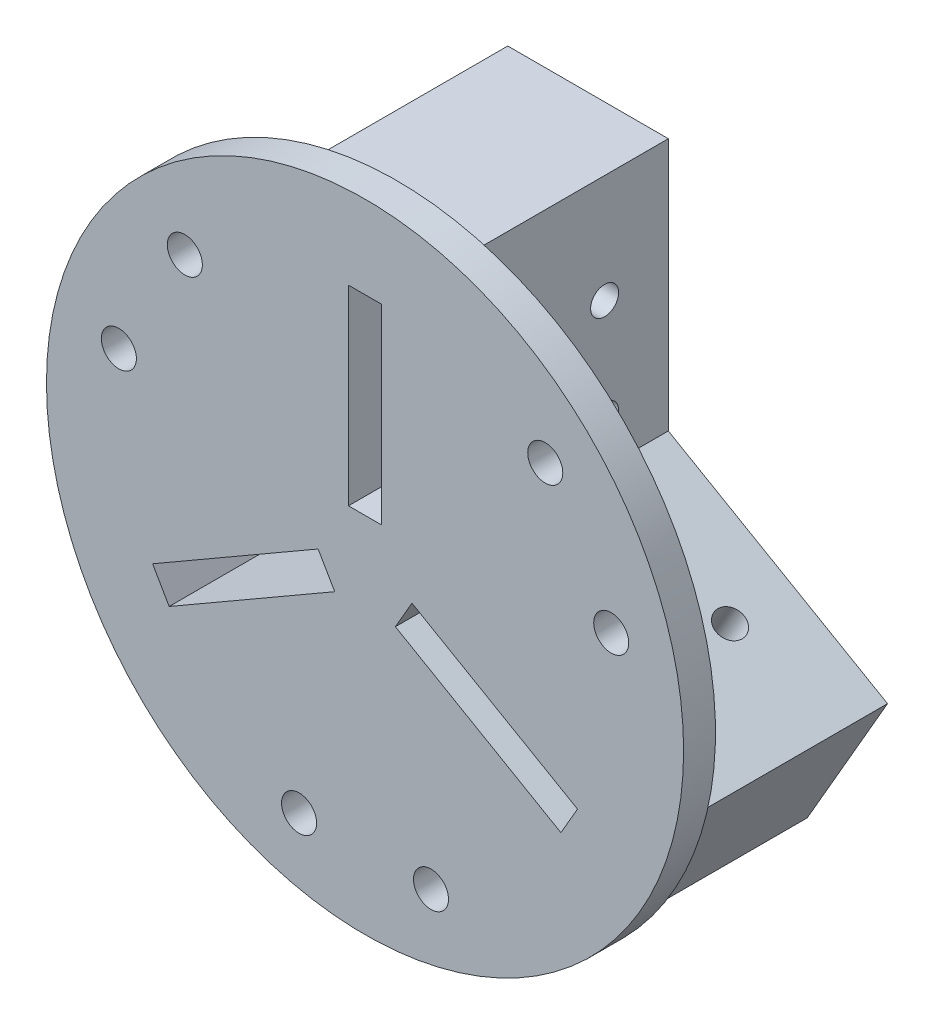
from build123d import *

# Parameters (mm, degrees)
SKETCH_1_R               = 50
SKETCH_1_W               = 5.2
SKETCH_1_H               = 30
EXTRUDE_1_DEPTH          = 5
SKETCH_2_R               = 60
SKETCH_2_W               = 5.2
SKETCH_2_H               = 30
EXTRUDE_2_DEPTH          = 10
CUT_EXTRUDE_START        = -10
SKETCH_4_R               = 60
CUT_EXTRUDE_1_DEPTH      = 10
SKETCH_8_W               = 5.2
SKETCH_8_H               = 30
EXTRUDE_5_DEPTH          = 20
SKETCH_6_R               = 2.2
CUT_EXTRUDE_2_DEPTH      = 42
PATTERN_CIRCULAR_1_COUNT = 3
SKETCH_9_R               = 2.75
CUT_EXTRUDE_3_DEPTH      = 10
SKETCH_10_R              = 6
CUT_EXTRUDE_4_DEPTH      = 0.5
PATTERN_CIRCULAR_2_COUNT = 3


with BuildPart() as part:
    # 草图1 → 凸台-拉伸1 (new body)
    with BuildSketch(Plane.XY):
        Circle(SKETCH_1_R)
        with Locations((0, 22)):
            Rectangle(SKETCH_1_W, SKETCH_1_H, mode=Mode.SUBTRACT)
        Polygon((4.762177826, -5.75166605), (30.74293994, -20.75166605), (33.34293994, -16.24833395), (7.362177826, -1.24833395), align=None, mode=Mode.SUBTRACT)
        Polygon((-7.362177826, -1.24833395), (-33.34293994, -16.24833395), (-30.74293994, -20.75166605), (-4.762177826, -5.75166605), align=None, mode=Mode.SUBTRACT)
    extrude(amount=EXTRUDE_1_DEPTH)

    # 草图2 → 凸台-拉伸2 (add)
    with BuildSketch(Plane.XY):
        Circle(SKETCH_2_R)
        with Locations((0, 22)):
            Rectangle(SKETCH_2_W, SKETCH_2_H, mode=Mode.SUBTRACT)
        Polygon((7.362177826, -1.24833395), (4.762177826, -5.75166605), (30.74293994, -20.75166605), (33.34293994, -16.24833395), align=None, mode=Mode.SUBTRACT)
        Polygon((-4.762177826, -5.75166605), (-7.362177826, -1.24833395), (-33.34293994, -16.24833395), (-30.74293994, -20.75166605), align=None, mode=Mode.SUBTRACT)
    extrude(amount=-EXTRUDE_2_DEPTH)

    # 草图4 → 切除-拉伸1 (cut)
    with BuildSketch(Plane(origin=(0, 0, -10), x_dir=(-1, 0, 0), z_dir=(0, 0, -1)).offset(CUT_EXTRUDE_START)):
        Circle(SKETCH_4_R)
        Polygon((-47.003193978, -12.588079912), (-12.6, 7.274613392), (-12.6, 47), (12.6, 47), (12.6, 7.274613392), (47.003193978, -12.588079912), (34.403193978, -34.411920088), (0, -14.549226784), (-34.403193978, -34.411920088), align=None, mode=Mode.SUBTRACT)
    extrude(amount=CUT_EXTRUDE_1_DEPTH, mode=Mode.SUBTRACT)

    # 草图8 → 凸台-拉伸5 (add)
    with BuildSketch(Plane(origin=(0, 0, -10), x_dir=(-1, 0, 0), z_dir=(0, 0, -1))):
        Polygon((47.003193978, -12.588079912), (12.6, 7.274613392), (12.6, 47), (-12.6, 47), (-12.6, 7.274613392), (-47.003193978, -12.588079912), (-34.403193978, -34.411920088), (0, -14.549226784), (34.403193978, -34.411920088), align=None)
        with Locations((0, 22)):
            Rectangle(SKETCH_8_W, SKETCH_8_H, mode=Mode.SUBTRACT)
        Polygon((-4.762177826, -5.75166605), (-7.362177826, -1.24833395), (-33.34293994, -16.24833395), (-30.74293994, -20.75166605), align=None, mode=Mode.SUBTRACT)
        Polygon((7.362177826, -1.24833395), (4.762177826, -5.75166605), (30.74293994, -20.75166605), (33.34293994, -16.24833395), align=None, mode=Mode.SUBTRACT)
    extrude(amount=EXTRUDE_5_DEPTH)

    # 草图6 → 切除-拉伸2 (cut)
    with BuildSketch(Plane(origin=(6.3, -10.911920088, 0), x_dir=(0.8660254037844384, 0.5000000000000004, 0), z_dir=(0.5000000000000004, -0.8660254037844384, 0))):
        with Locations((-30, -20)):
            Circle(SKETCH_6_R)
        with Locations((-14, -20)):
            Circle(SKETCH_6_R)
    cut_extrude_2 = extrude(amount=-CUT_EXTRUDE_2_DEPTH, mode=Mode.SUBTRACT)

    # 阵列(圆周)1: 切除-拉伸2 ×3 about axis
    pattern_circular_1_axis = Axis((0, 0, 5), (0, 0, -1))
    for i in range(1, PATTERN_CIRCULAR_1_COUNT):
        add(cut_extrude_2.rotate(pattern_circular_1_axis, i * 360 / PATTERN_CIRCULAR_1_COUNT), mode=Mode.SUBTRACT)

    # 草图9 → 切除-拉伸3 (cut)
    with BuildSketch(Plane(origin=(0, 0, 0), x_dir=(-1, 0, 0), z_dir=(0, 0, -1))):
        with Locations((28.284271247, 28.284271247)):
            Circle(SKETCH_9_R)
        with Locations((38.637033052, 10.352761804)):
            Circle(SKETCH_9_R)
    cut_extrude_3 = extrude(amount=-CUT_EXTRUDE_3_DEPTH, mode=Mode.SUBTRACT)

    # 草图10 → 切除-拉伸4 (cut)
    with BuildSketch(Plane(origin=(0, 0, 0), x_dir=(-1, 0, 0), z_dir=(0, 0, -1))):
        with Locations((28.284271247, 28.284271247)):
            Circle(SKETCH_10_R)
        with Locations((38.637033052, 10.352761804)):
            Circle(SKETCH_10_R)
    cut_extrude_4 = extrude(amount=-CUT_EXTRUDE_4_DEPTH, mode=Mode.SUBTRACT)

    # 阵列(圆周)2: 切除-拉伸3, 切除-拉伸4 ×3 about axis
    pattern_circular_2_axis = Axis((0, 0, 0), (0, 0, 1))
    add([cut_extrude_3.rotate(pattern_circular_2_axis, i * 360 / PATTERN_CIRCULAR_2_COUNT) for i in range(1, PATTERN_CIRCULAR_2_COUNT)], mode=Mode.SUBTRACT)
    add([cut_extrude_4.rotate(pattern_circular_2_axis, i * 360 / PATTERN_CIRCULAR_2_COUNT) for i in range(1, PATTERN_CIRCULAR_2_COUNT)], mode=Mode.SUBTRACT)


solid = part.part
